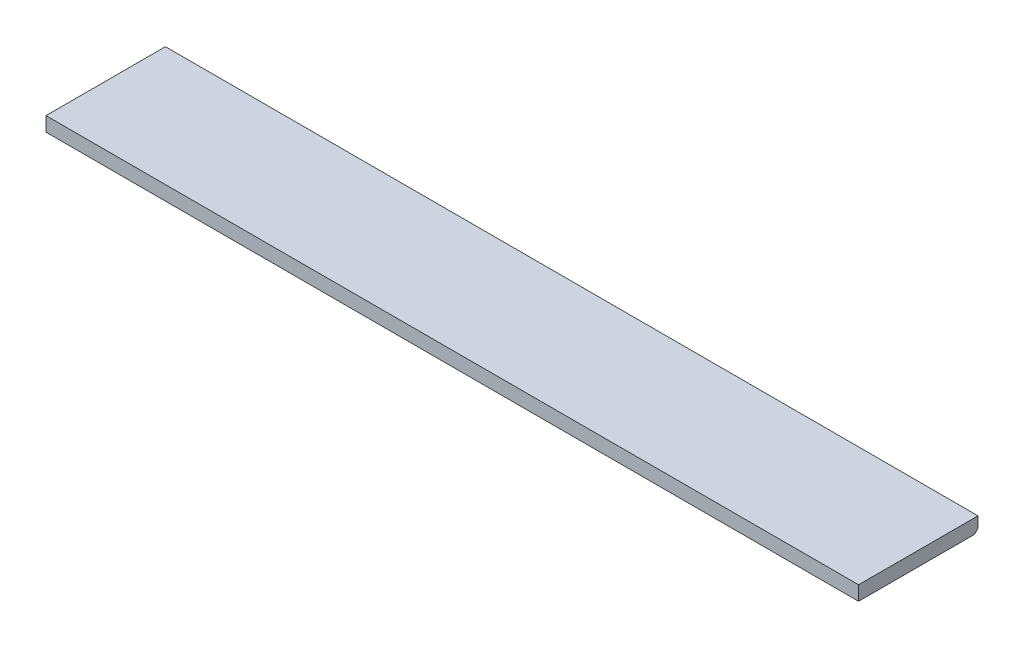
SolidWorks part; units mm, degrees
ref_plane "前视基准面" through (0, 0, 0) normal (0, 0, 1) x (1, 0, 0)
ref_plane "上视基准面" through (0, 0, 0) normal (0, 1, 0) x (1, 0, 0)
ref_plane "右视基准面" through (0, 0, 0) normal (1, 0, 0) x (0, 0, -1)
sketch "草图1" plane through (0, 0, 0) normal (0, 1, 0) x (1, 0, 0)
  line L1 (-1133, -166.5) -> (1133, -166.5)
  line L2 (-1133, -166.5) -> (-1133, 166.5)
  line L3 (-1133, 166.5) -> (1133, 166.5)
  line L4 (1133, -166.5) -> (1133, 166.5)
  line L5 (-1133, -166.5) -> (1133, 166.5) construction
  line L6 (-1133, 166.5) -> (1133, -166.5) construction
  point P0 (0, 0)
  dimension "D1" = 333
  dimension "D2" = 2266
extrude "凸台-拉伸1" add sketch "草图1" along normal blind 40
chamfer "倒角1" distance 10 angle 45 1 edges at (0, 0, -166.5)
